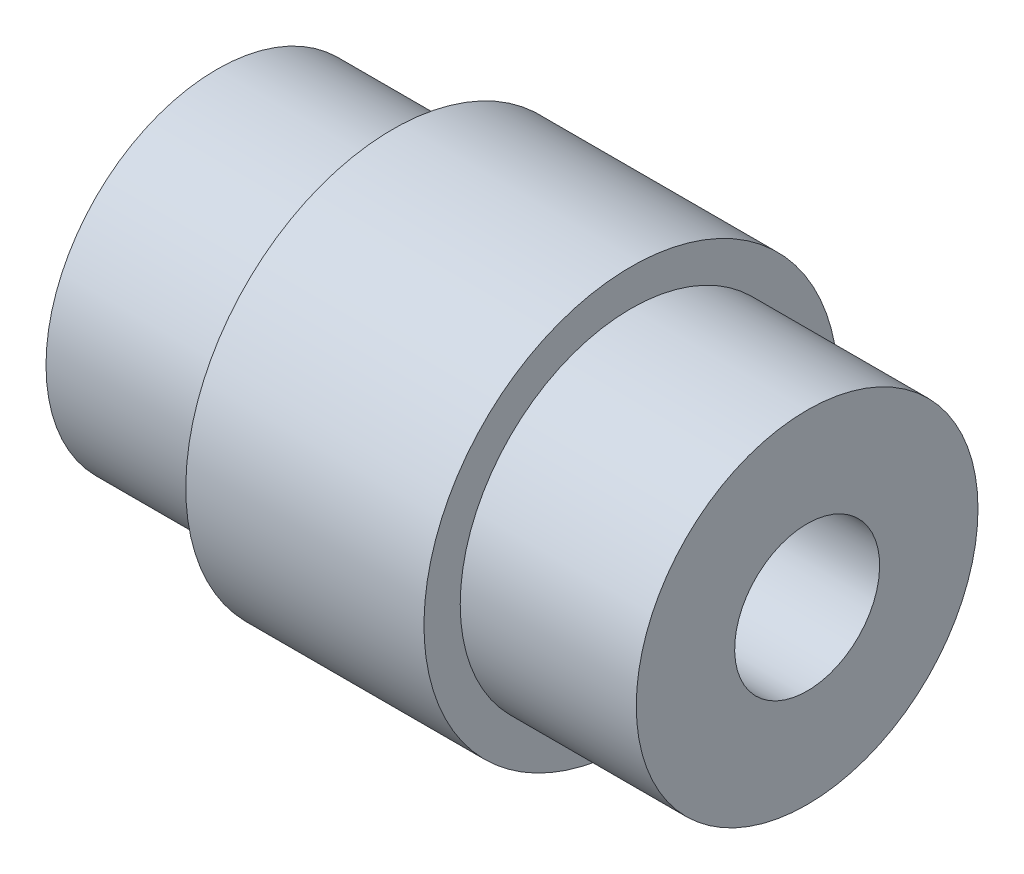
from build123d import *

# Parameters (mm, degrees)
SKETCH_2_R          = 11
CUT_EXTRUDE_1_DEPTH = 45
SKETCH_3_R          = 14
CUT_EXTRUDE_2_DEPTH = 45


with BuildPart() as part:
    # 草图1 → 旋转1 (revolve)
    with BuildSketch(Plane.XY, mode=Mode.PRIVATE) as revolve_1_sk:
        Polygon((-57, -7.291938998), (57, -7.291938998), (57, 25.708061002), (23, 25.708061002), (23, 32.708061002), (-23, 32.708061002), (-23, 25.708061002), (-57, 25.708061002), align=None)
    revolve(revolve_1_sk.sketch.rotate(Axis((-57, -7.291938998, 0), (1, 0, 0)), 180), axis=Axis((-57, -7.291938998, 0), (1, 0, 0)))

    # 草图2 → 切除-拉伸1 (cut)
    with BuildSketch(Plane.ZY.offset(57)):
        with Locations(Location((0, -7.291938998, 0), (0, 0, 270))):
            Circle(SKETCH_2_R)
    extrude(amount=-CUT_EXTRUDE_1_DEPTH, mode=Mode.SUBTRACT)

    # 草图3 → 切除-拉伸2 (cut)
    with BuildSketch(Plane(origin=(57, 0, 0), x_dir=(0, 0, -1), z_dir=(1, 0, 0))):
        with Locations(Location((0, -7.291938998, 0), (0, 0, 90))):
            Circle(SKETCH_3_R)
    extrude(amount=-CUT_EXTRUDE_2_DEPTH, mode=Mode.SUBTRACT)


solid = part.part
